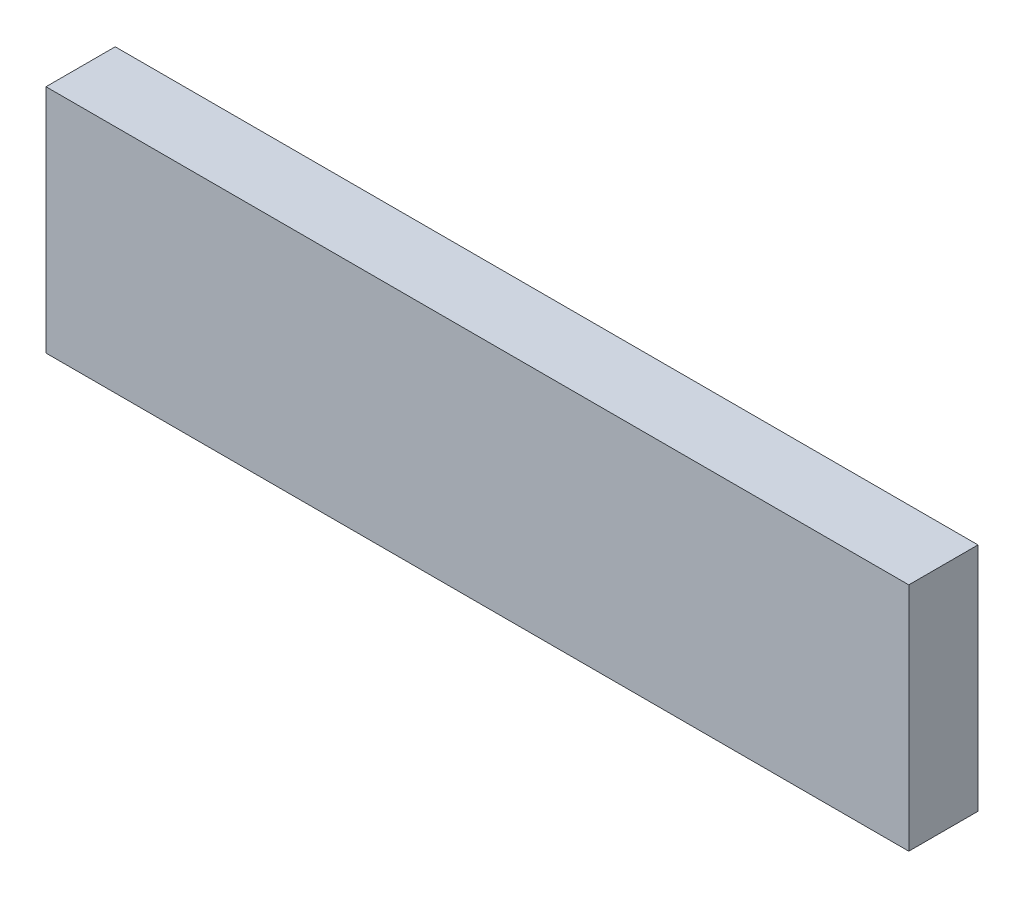
SolidWorks part; units mm, degrees
material "1023 碳钢板 (SS)"
ref_plane "前视基准面" through (0, 0, 0) normal (0, 0, 1) x (1, 0, 0)
ref_plane "上视基准面" through (0, 0, 0) normal (0, 1, 0) x (1, 0, 0)
ref_plane "右视基准面" through (0, 0, 0) normal (1, 0, 0) x (0, 0, -1)
sketch "草图1" plane through (0, 0, 0) normal (0, 0, 1) x (1, 0, 0)
  line L1 (93.5, 25) -> (-93.5, 25)
  line L2 (93.5, 25) -> (93.5, -25)
  line L3 (93.5, -25) -> (-93.5, -25)
  line L4 (-93.5, 25) -> (-93.5, -25)
  line L5 (93.5, 25) -> (-93.5, -25) construction
  line L6 (93.5, -25) -> (-93.5, 25) construction
  point P0 (0, 0)
  dimension "D1" = 187
  dimension "D2" = 50
extrude "凸台-拉伸1" add sketch "草图1" along normal blind 15
